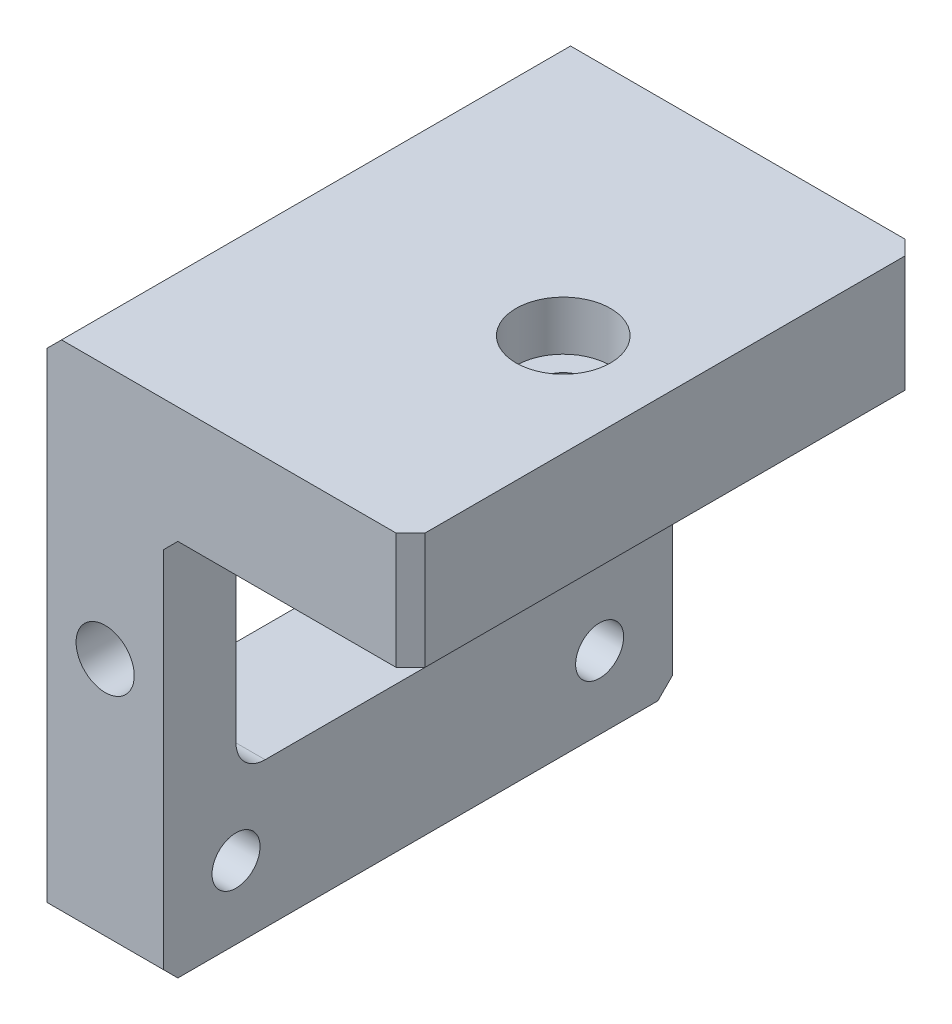
from build123d import *

# Parameters (mm, degrees)
BOSS_EXTRUDE1_DEPTH                                 = 17.5
SKETCH2_W                                           = 25
SKETCH2_H                                           = 15
CUT_EXTRUDE1_DEPTH                                  = 47.435439053
M4_TAPPED_HOLE1_D                                   = 3.3
M4_TAPPED_HOLE1_DEPTH                               = 11.5
M4_TAPPED_HOLE1_TIP                                 = 0.991420021
SKETCH5_R                                           = 2
CUT_EXTRUDE2_DEPTH                                  = 56.452682532
FILLET1_R                                           = 2
SKETCH6_R                                           = 4
CUT_EXTRUDE3_DEPTH                                  = 3
CHAMFER1_SIZE                                       = 1
CBORE_FOR_M3_HEX_SOCKET_HEAD_CAP_SCREW1_D           = 3.4
CBORE_FOR_M3_HEX_SOCKET_HEAD_CAP_SCREW1_CBORE_D     = 6.5
CBORE_FOR_M3_HEX_SOCKET_HEAD_CAP_SCREW1_CBORE_DEPTH = 3.4


with BuildPart() as part:
    # Sketch1 → Boss-Extrude1 (new, symmetric)
    with BuildSketch(Plane.XY):
        Polygon((0, 0), (0, 35), (25, 35), (25, 27), (8, 27), (8, 0), align=None)
    extrude(amount=BOSS_EXTRUDE1_DEPTH, both=True)

    # Sketch2 → Cut-Extrude1 (cut, through all)
    with BuildSketch(Plane.ZY):
        with Locations((0, 17.5)):
            Rectangle(SKETCH2_W, SKETCH2_H)
    extrude(amount=-CUT_EXTRUDE1_DEPTH, mode=Mode.SUBTRACT)

    # M4 Tapped Hole1
    with Locations(Plane.ZY):
        with Locations((-12.5, 5), (12.5, 5)):
            Hole(M4_TAPPED_HOLE1_D / 2, depth=M4_TAPPED_HOLE1_DEPTH)
            with Locations((0, 0, -(M4_TAPPED_HOLE1_DEPTH + M4_TAPPED_HOLE1_TIP / 2))):  # 118° drill point
                Cone(0, M4_TAPPED_HOLE1_D / 2, M4_TAPPED_HOLE1_TIP, mode=Mode.SUBTRACT)

    # Sketch5 → Cut-Extrude2 (cut, through all)
    with BuildSketch(Plane.XY.offset(17.5)):
        with Locations((4, 17.5)):
            Circle(SKETCH5_R)
    extrude(amount=-CUT_EXTRUDE2_DEPTH, mode=Mode.SUBTRACT)

    # Fillet1
    fillet1_edges = [part.edges().sort_by_distance(p)[0] for p in [
        (4, 10, -12.5),
        (4, 25, -12.5),
        (4, 25, 12.5),
        (4, 10, 12.5),
    ]]
    fillet(fillet1_edges, radius=FILLET1_R)

    # Sketch6 → Cut-Extrude3 (cut)
    with BuildSketch(Plane.XZ.offset(-27)):
        with Locations((18, 0)):
            Circle(SKETCH6_R)
    extrude(amount=-CUT_EXTRUDE3_DEPTH, mode=Mode.SUBTRACT)

    # Chamfer1
    chamfer1_edges = [part.edges().sort_by_distance(p)[0] for p in [
        (0, 35, 0),
        (8, 27, 0),
        (25, 31, 17.5),
        (4, 0, 17.5),
        (25, 31, -17.5),
        (4, 0, -17.5),
    ]]
    chamfer(chamfer1_edges, length=CHAMFER1_SIZE)

    # CBORE for M3 Hex Socket Head Cap Screw1 (through all)
    with Locations(Plane(origin=(0, 35, 0), x_dir=(1, 0, 0), z_dir=(0, 1, 0))):
        with Locations((18, 0)):
            CounterBoreHole(CBORE_FOR_M3_HEX_SOCKET_HEAD_CAP_SCREW1_D / 2, CBORE_FOR_M3_HEX_SOCKET_HEAD_CAP_SCREW1_CBORE_D / 2, CBORE_FOR_M3_HEX_SOCKET_HEAD_CAP_SCREW1_CBORE_DEPTH)


solid = part.part
